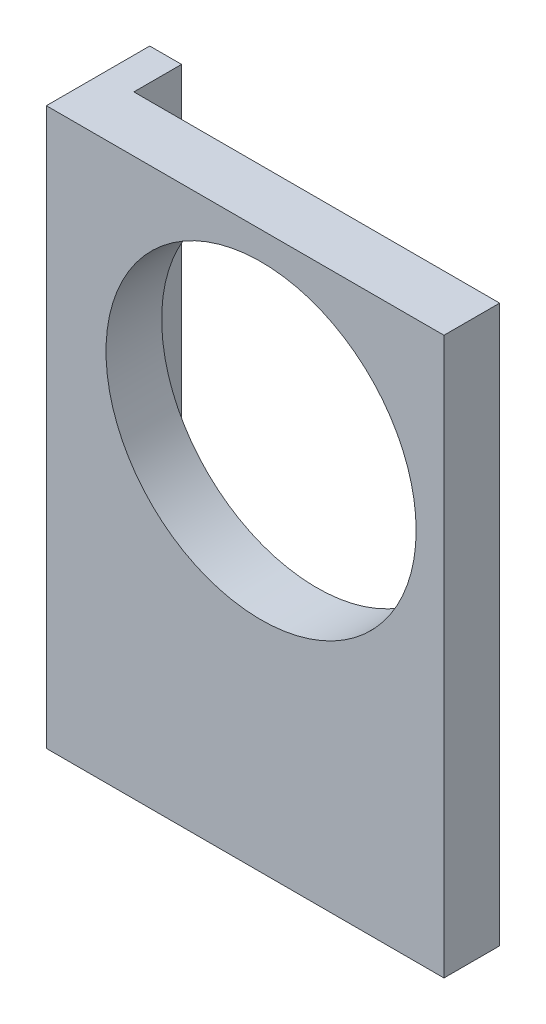
SolidWorks part; units mm, degrees
ref_plane "前视基准面" through (0, 0, 0) normal (0, 0, 1) x (1, 0, 0)
ref_plane "上视基准面" through (0, 0, 0) normal (0, 1, 0) x (1, 0, 0)
ref_plane "右视基准面" through (0, 0, 0) normal (1, 0, 0) x (0, 0, -1)
sketch "草图1" plane through (0, 0, 0) normal (0, 0, 1) x (1, 0, 0)
  line L1 (-50, -70) -> (50, -70)
  line L2 (-50, -70) -> (-50, 70)
  line L3 (-50, 70) -> (50, 70)
  line L4 (50, -70) -> (50, 70)
  line L5 (-50, -70) -> (50, 70) construction
  line L6 (-50, 70) -> (50, -70) construction
  point P0 (0, 0)
  dimension "D1" = 100
  dimension "D2" = 140
extrude "凸台-拉伸1" add sketch "草图1" along normal blind 14
sketch "草图2" plane through (0, 0, 14) normal (0, 0, 1) x (1, 0, 0)
  line L0 (50, 70) -> (-50, 70) construction
  line L1 (50, -70) -> (50, 70) construction
  circle A0 centre (4, 24) radius 39
  dimension "D1" = 78
  dimension "D2" = 46
  dimension "D3" = 46
extrude "切除-拉伸1" cut sketch "草图2" against normal up to next
sketch "草图3" plane through (0, 0, 0) normal (0, 0, 1) x (1, 0, 0)
  line L0 (-50, -70) -> (50, -70) construction
  line L1 (-50, 70) -> (-42, 70)
  line L2 (-50, 70) -> (-50, -70)
  line L3 (-50, -70) -> (-42, -70)
  line L4 (-42, 70) -> (-42, -70)
  dimension "D1" = 8
extrude "凸台-拉伸2" add sketch "草图3" against normal blind 12
